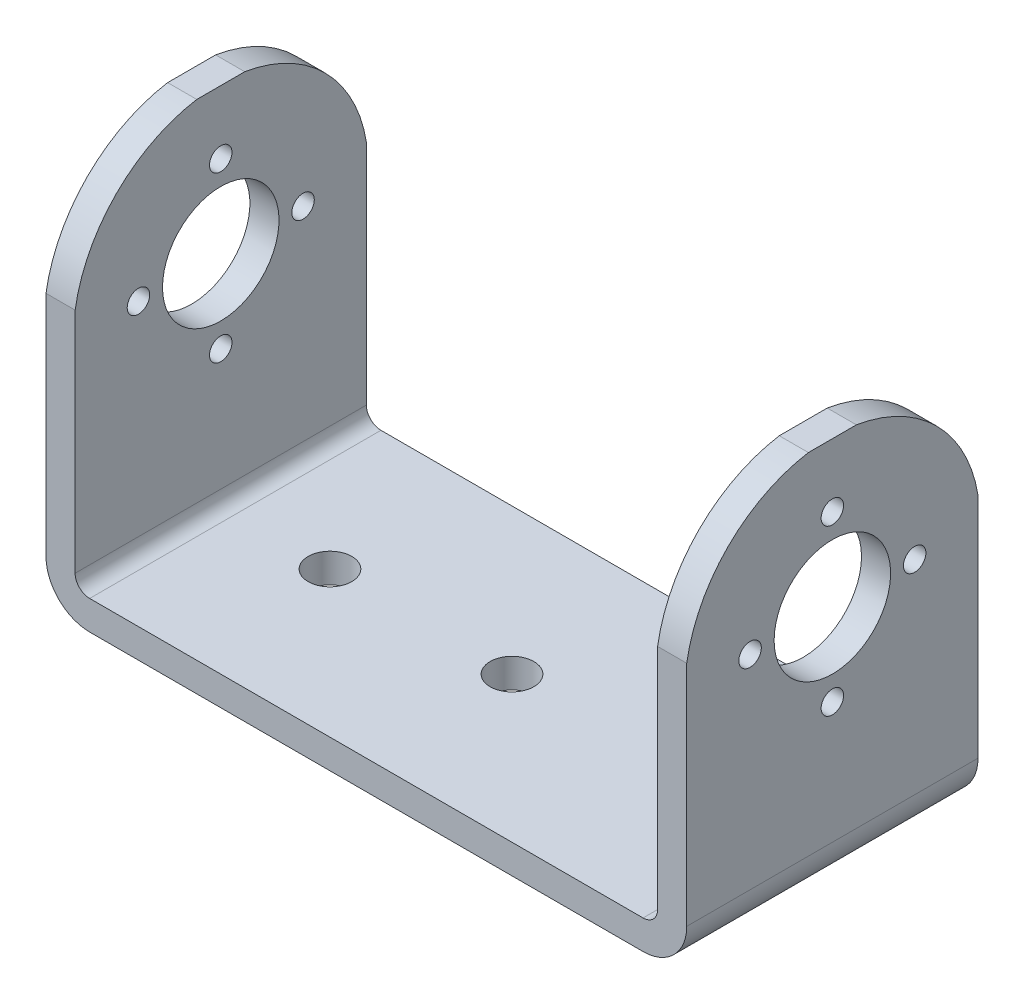
from build123d import *

# Parameters (mm, degrees)
BOSS_EXTRUDE1_DEPTH = 20
SKETCH2_R           = 4
SKETCH2_R_2         = 0.771303816
CUT_EXTRUDE1_DEPTH  = 55.415071442
SKETCH3_R           = 1.5
CUT_EXTRUDE2_DEPTH  = 53.810983706


with BuildPart() as part:
    # Sketch1 → Boss-Extrude1 (new body)
    with BuildSketch(Plane.XY):
        with BuildLine():
            Line((0, 25), (0, 1))
            ThreePointArc((0, 1), (0.292893219, 0.292893219), (1, 0))
            Line((1, 0), (39, 0))
            ThreePointArc((39, 0), (39.707106781, 0.292893219), (40, 1))
            Line((40, 1), (40, 25))
            Line((40, 25), (42, 25))
            Line((42, 25), (42, 1))
            ThreePointArc((42, 1), (41.121320344, -1.121320344), (39, -2))
            Line((39, -2), (1, -2))
            ThreePointArc((1, -2), (-1.121320344, -1.121320344), (-2, 1))
            Line((-2, 1), (-2, 25))
            Line((-2, 25), (0, 25))
        make_face()
    extrude(amount=BOSS_EXTRUDE1_DEPTH)

    # Sketch2 → Cut-Extrude1 (cut, through all)
    with BuildSketch(Plane.ZY.offset(2)):
        with Locations((10, 15)):
            Circle(SKETCH2_R)
        with Locations((10, 20.651236345)):
            Circle(SKETCH2_R_2)
        with Locations((15.651236345, 15)):
            Circle(SKETCH2_R_2)
        with Locations((10, 9.348763655)):
            Circle(SKETCH2_R_2)
        with Locations((4.348763655, 15)):
            Circle(SKETCH2_R_2)
        with BuildLine():
            Line((-0.134788382, 15), (-9.479992385, 25.134788382))
            Line((-9.479992385, 25.134788382), (9.199881334, 33.71105644))
            Line((9.199881334, 33.71105644), (31.219173818, 26.927862072))
            Line((31.219173818, 26.927862072), (20.134788382, 15))
            ThreePointArc((20.134788382, 15), (10, 25.134788382), (-0.134788382, 15))
        make_face()
    extrude(amount=-CUT_EXTRUDE1_DEPTH, mode=Mode.SUBTRACT)

    # Sketch3 → Cut-Extrude2 (cut, through all)
    with BuildSketch(Plane(origin=(0, 0, 0), x_dir=(1, 0, 0), z_dir=(0, 1, 0))):
        with Locations(Location((7.5, -10, 0), (0, 0, 270))):
            Circle(SKETCH3_R)
        with Locations(Location((20, -10, 0), (0, 0, 270))):
            Circle(SKETCH3_R)
        with Locations(Location((32.5, -10, 0), (0, 0, 270))):
            Circle(SKETCH3_R)
    extrude(amount=-CUT_EXTRUDE2_DEPTH, mode=Mode.SUBTRACT)


solid = part.part
